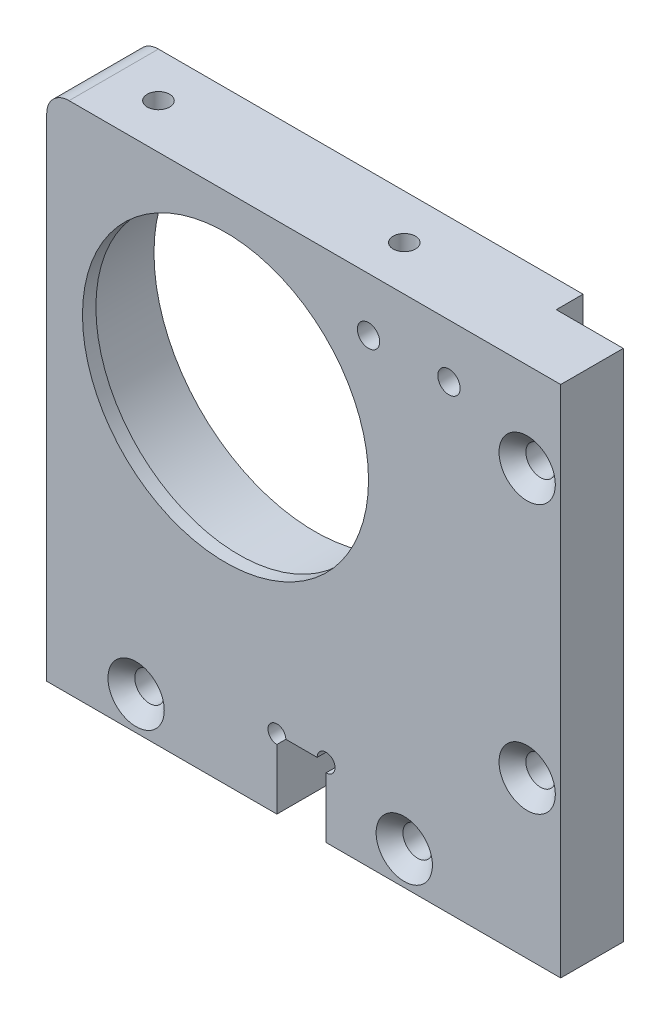
from build123d import *

# Parameters (mm, degrees)
SKETCH_1_W                   = 115
SKETCH_1_H                   = 115
EXTRUDE_1_DEPTH              = 20
CUT_EXTRUDE_1_DEPTH          = 6
SKETCH_3_R                   = 32
CUT_EXTRUDE_2_DEPTH          = 84.740671122
SKETCH_4_R                   = 36
CUT_EXTRUDE_3_DEPTH          = 17
SKETCH_5_W                   = 11
SKETCH_5_H                   = 15.5
CUT_EXTRUDE_4_DEPTH          = 84.740671122
SKETCH_6_R                   = 2
CUT_EXTRUDE_5_DEPTH          = 84.740671122
HOLE_WIZARD_M6_1_D           = 6.6
HOLE_WIZARD_M6_1_CSINK_D     = 12.6
HOLE_WIZARD_M6_1_CSINK_ANGLE = 90
FILLET_1_R                   = 5
HOLE_WIZARD_M6_1_2_D         = 5
HOLE_WIZARD_M6_1_2_DEPTH     = 17
HOLE_WIZARD_M6_1_2_TIP       = 1.502151548
HOLE_WIZARD_M6_2_D           = 5
HOLE_WIZARD_M6_2_DEPTH       = 17
HOLE_WIZARD_M6_2_TIP         = 1.502151548


with BuildPart() as part:
    # 草图1 → 凸台-拉伸1 (new body)
    with BuildSketch(Plane.XY):
        Rectangle(SKETCH_1_W, SKETCH_1_H)
    extrude(amount=EXTRUDE_1_DEPTH)

    # 草图2 → 切除-拉伸1 (cut)
    with BuildSketch(Plane(origin=(0, 0, 0), x_dir=(-1, 0, 0), z_dir=(0, 0, -1))):
        Polygon((-57.5, 57.5), (-42.5, 57.5), (-42.5, -42.5), (57.5, -42.5), (57.5, -57.5), (-57.5, -57.5), align=None)
    extrude(amount=-CUT_EXTRUDE_1_DEPTH, mode=Mode.SUBTRACT)

    # 草图3 → 切除-拉伸2 (cut, through all)
    with BuildSketch(Plane(origin=(0, 0, 0), x_dir=(-1, 0, 0), z_dir=(0, 0, -1))):
        with Locations((17.5, 17.5)):
            Circle(SKETCH_3_R)
    extrude(amount=-CUT_EXTRUDE_2_DEPTH, mode=Mode.SUBTRACT)

    # 草图4 → 切除-拉伸3 (cut)
    with BuildSketch(Plane(origin=(0, 0, 0), x_dir=(-1, 0, 0), z_dir=(0, 0, -1))):
        with Locations((17.5, 17.5)):
            Circle(SKETCH_4_R)
    extrude(amount=-CUT_EXTRUDE_3_DEPTH, mode=Mode.SUBTRACT)

    # 草图5 → 切除-拉伸4 (cut, through all)
    with BuildSketch(Plane.XY.offset(20)):
        with Locations((-0.5, -49.75)):
            Rectangle(SKETCH_5_W, SKETCH_5_H)
    extrude(amount=-CUT_EXTRUDE_4_DEPTH, mode=Mode.SUBTRACT)

    # 草图6 → 切除-拉伸5 (cut, through all)
    with BuildSketch(Plane.XY.offset(20)):
        with Locations((-6, -42)):
            Circle(SKETCH_6_R)
        with Locations((5, -42)):
            Circle(SKETCH_6_R)
    extrude(amount=-CUT_EXTRUDE_5_DEPTH, mode=Mode.SUBTRACT)

    # Hole Wizard M6 _1 (through all)
    with Locations(Plane.XY.offset(20)):
        with Locations((-37.5, -50), (22.5, -50), (50, -22.5), (50, 37.5)):
            CounterSinkHole(HOLE_WIZARD_M6_1_D / 2, HOLE_WIZARD_M6_1_CSINK_D / 2, counter_sink_angle=HOLE_WIZARD_M6_1_CSINK_ANGLE)

    # 圆角1
    fillet_1_edges = [part.edges().sort_by_distance(p)[0] for p in [
        (-57.5, 57.5, 10),
    ]]
    fillet(fillet_1_edges, radius=FILLET_1_R)

    # Hole Wizard M6 _1 2
    with Locations(Plane.XY.offset(20)):
        with Locations((32.5, 45.5), (14.5, 45.5)):
            Hole(HOLE_WIZARD_M6_1_2_D / 2, depth=HOLE_WIZARD_M6_1_2_DEPTH)
            with Locations((0, 0, -(HOLE_WIZARD_M6_1_2_DEPTH + HOLE_WIZARD_M6_1_2_TIP / 2))):  # 118° drill point
                Cone(0, HOLE_WIZARD_M6_1_2_D / 2, HOLE_WIZARD_M6_1_2_TIP, mode=Mode.SUBTRACT)

    # M6 螺纹孔2
    with Locations(Plane(origin=(0, 57.5, 0), x_dir=(1, 0, 0), z_dir=(0, 1, 0))):
        with Locations((-42.5, -10), (12.5, -10)):
            Hole(HOLE_WIZARD_M6_2_D / 2, depth=HOLE_WIZARD_M6_2_DEPTH)
            with Locations((0, 0, -(HOLE_WIZARD_M6_2_DEPTH + HOLE_WIZARD_M6_2_TIP / 2))):  # 118° drill point
                Cone(0, HOLE_WIZARD_M6_2_D / 2, HOLE_WIZARD_M6_2_TIP, mode=Mode.SUBTRACT)


solid = part.part
